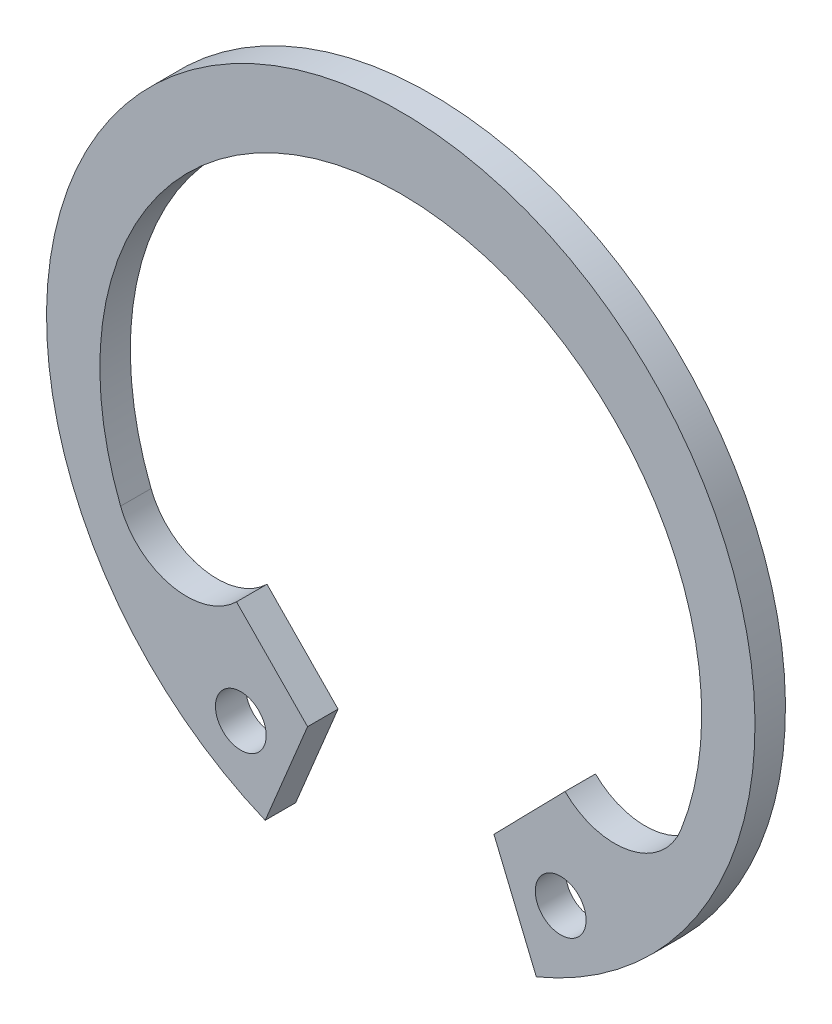
SolidWorks part; units mm, degrees
ref_plane "前视" through (0, 0, 0) normal (0, 0, 1) x (1, 0, 0)
ref_plane "上视" through (0, 0, 0) normal (0, 1, 0) x (1, 0, 0)
ref_plane "右视" through (0, 0, 0) normal (1, 0, 0) x (0, 0, -1)
sketch "草图1" plane through (0, 0, 0) normal (0, 0, 1) x (1, 0, 0)
  line L0 (0, -11.8766) -> (0, 11.8063) construction
  line L1 (0, 0) -> (-4.6199, -11.1535) construction
  line L2 (-6.468, -6.0015) -> (-3.6699, -8.86)
  line L3 (-3.6699, -8.86) -> (-5.3384, -12.8881)
  line L4 (3.6699, -8.86) -> (5.3384, -12.8881)
  line L5 (6.468, -6.0015) -> (3.6699, -8.86)
  arc A0 (5.3384, -12.8881) -> (-5.3384, -12.8881) centre (0, 0) ccw
  arc A1 (11.0338, -5.0218) -> (-11.0338, -5.0218) centre (0, -0.7) ccw
  circle A2 centre (-6.2981, -9.9787) radius 1
  arc A3 (-11.0338, -5.0218) -> (-6.468, -6.0015) centre (-8.4267, -4.0006) ccw
  circle A4 centre (6.2981, -9.9787) radius 1
  arc A5 (11.0338, -5.0218) -> (6.468, -6.0015) centre (8.4267, -4.0006) cw
sketch "尺寸草图" plane through (0, 0, 0) normal (0, 0, 1) x (1, 0, 0)
  line L0 (-13.95, 0) -> (13.95, 0) construction
  line L1 (0, 0) -> (29.4981, -33.9833) construction
  circle A2 centre (0, 0) radius 13.95
  point P9 (9.75, 0)
  point P10 (10.45, 0)
  point P11 (-9, 0)
  point P12 (-5.8, 0)
  point P13 (4.36, 0)
  point P14 (-9.8, 0)
  point P15 (-13.8, 0)
  point P16 (-11.8, 0)
  point P18 (0.7866, -0.9062)
extrude "基体-拉伸" add sketch "草图1" along normal blind 1.2
equation "\"D1@草图1\" = \"DD@尺寸草图\""
equation "\"D2@草图1\" = \"d@尺寸草图\""
equation "\"D5@草图1\" = \"R2@尺寸草图\""
equation "\"D9@草图1\" = \"R@尺寸草图\""
equation "\"D7@草图1\" = \"B@尺寸草图\""
equation "\"D10@草图1\" = \"B1@尺寸草图\""
equation "\"D4@草图1\" = \"d1@尺寸草图\""
equation "\"D6@草图1\" = \"a@尺寸草图\""
equation "\"D8@草图1\" = \"aa@尺寸草图\"/2"
equation "\"D3@草图1\" = \"c@尺寸草图\""
equation "\"D1@基体-拉伸\"=\"s@尺寸草图\"/2"
equation "\"D2@基体-拉伸\" = \"D1@基体-拉伸\""
